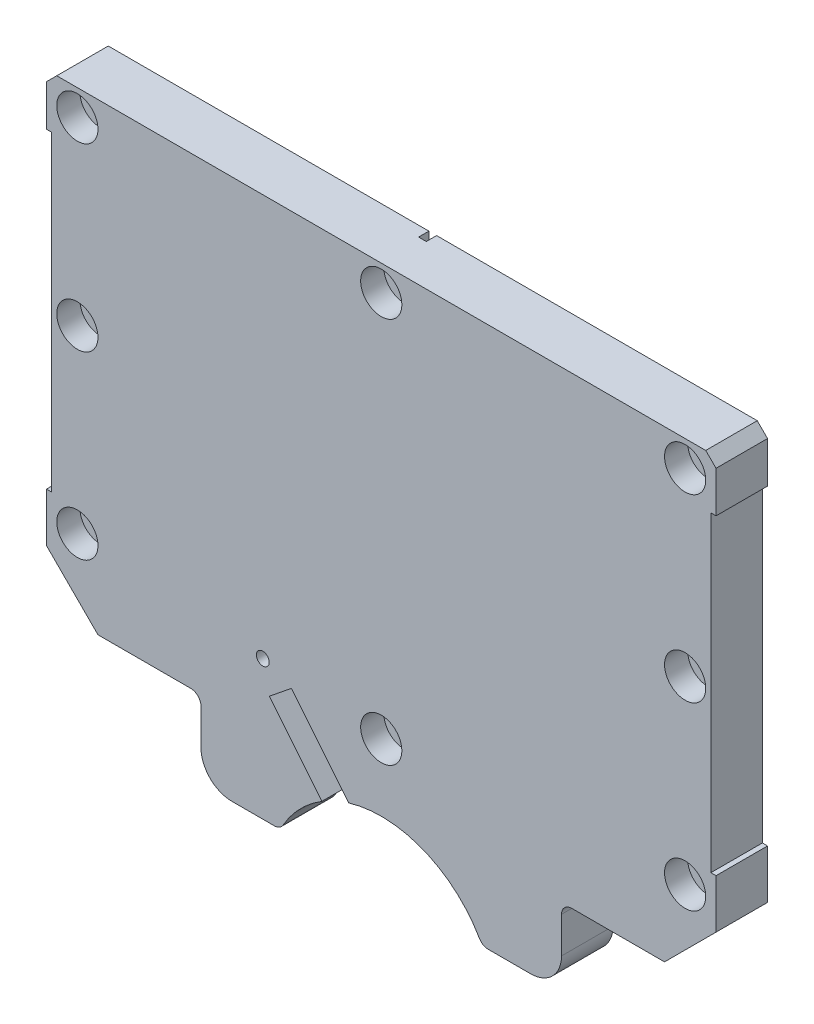
from build123d import *

# Parameters (mm, degrees)
SKETCH1_W                                            = 130
SKETCH1_H                                            = 105
BOSS_EXTRUDE1_DEPTH                                  = 5
SKETCH3_R                                            = 22
CUT_EXTRUDE2_DEPTH                                   = 85.150163399
SKETCH7_W                                            = 30
SKETCH7_H                                            = 10
CUT_EXTRUDE5_DEPTH                                   = 15
FILLET1_R                                            = 6
CHAMFER1_SIZE                                        = 10
FILLET2_R                                            = 2
CUT_EXTRUDE8_DEPTH                                   = 85.150163399
FILLET3_R                                            = 2
CHAMFER2_SIZE                                        = 2
SKETCH15_W                                           = 1
SKETCH15_H                                           = 60.5
CUT_EXTRUDE10_DEPTH                                  = 85.150163399
HOLE_SIZE_PER_SOCKET_HEAD_CAP_SCREW_TYPE_D           = 4.5
HOLE_SIZE_PER_SOCKET_HEAD_CAP_SCREW_TYPE_CBORE_D     = 8
HOLE_SIZE_PER_SOCKET_HEAD_CAP_SCREW_TYPE_CBORE_DEPTH = 4.5
M3_TAPPED_HOLE1_D                                    = 2.5
M3_TAPPED_HOLE1_DEPTH                                = 8.5
M3_TAPPED_HOLE1_TIP                                  = 0.751075774
SKETCH20_W                                           = 1.5
SKETCH20_H                                           = 105
CUT_EXTRUDE11_DEPTH                                  = 2


with BuildPart() as part:
    # Sketch1 → Boss-Extrude1 (new, symmetric)
    with BuildSketch(Plane.XY):
        Rectangle(SKETCH1_W, SKETCH1_H)
    extrude(amount=BOSS_EXTRUDE1_DEPTH, both=True)

    # Sketch3 → Cut-Extrude2 (cut, through all)
    with BuildSketch(Plane.XY.offset(5)):
        with Locations((0, -62.5)):
            Circle(SKETCH3_R)
    extrude(amount=-CUT_EXTRUDE2_DEPTH, mode=Mode.SUBTRACT)

    # Sketch7 → Cut-Extrude5 (cut)
    with BuildSketch(Plane.XZ.offset(52.5)):
        with Locations((-50, 0)):
            Rectangle(SKETCH7_W, SKETCH7_H)
        with Locations((50, 0)):
            Rectangle(SKETCH7_W, SKETCH7_H)
    extrude(amount=-CUT_EXTRUDE5_DEPTH, mode=Mode.SUBTRACT)

    # Fillet1
    fillet1_edges = [part.edges().sort_by_distance(p)[0] for p in [
        (-35, -52.5, 0),
        (35, -52.5, 0),
    ]]
    fillet(fillet1_edges, radius=FILLET1_R)

    # Chamfer1
    chamfer1_edges = [part.edges().sort_by_distance(p)[0] for p in [
        (-65, -37.5, 0),
        (65, -37.5, 0),
    ]]
    chamfer(chamfer1_edges, length=CHAMFER1_SIZE)

    # Fillet2
    fillet2_edges = [part.edges().sort_by_distance(p)[0] for p in [
        (-35, -37.5, 0),
        (35, -37.5, 0),
    ]]
    fillet(fillet2_edges, radius=FILLET2_R)

    # Sketch10 → Cut-Extrude8 (cut, through all)
    with BuildSketch(Plane.XY.offset(5)):
        Polygon((-21.710710609, -31.184123297), (-17.436407821, -27.722861146), (-4.85, -43.265780375), (-9.124302788, -46.727042526), align=None)
    extrude(amount=-CUT_EXTRUDE8_DEPTH, mode=Mode.SUBTRACT)

    # Fillet3
    fillet3_edges = [part.edges().sort_by_distance(p)[0] for p in [
        (-19.595917942, -52.5, 0),
        (19.595917942, -52.5, 0),
    ]]
    fillet(fillet3_edges, radius=FILLET3_R)

    # Chamfer2
    chamfer2_edges = [part.edges().sort_by_distance(p)[0] for p in [
        (-65, 52.5, 0),
        (65, 52.5, 0),
    ]]
    chamfer(chamfer2_edges, length=CHAMFER2_SIZE)

    # Sketch15 → Cut-Extrude10 (cut, through all)
    with BuildSketch(Plane(origin=(0, 0, -5), x_dir=(-1, 0, 0), z_dir=(0, 0, -1))):
        with Locations((-64.5, 12.25)):
            Rectangle(SKETCH15_W, SKETCH15_H)
        with Locations((64.5, 12.25)):
            Rectangle(SKETCH15_W, SKETCH15_H)
    extrude(amount=-CUT_EXTRUDE10_DEPTH, mode=Mode.SUBTRACT)

    # Hole size per socket head cap screw type 0 (through all)
    with Locations(Plane.XY.offset(5)):
        with Locations((59, 47.5), (0, 47.5), (-59, 47.5), (-59, 12.5), (-59, -22.5), (0, -27.5), (59, -22.5), (59, 12.5)):
            CounterBoreHole(HOLE_SIZE_PER_SOCKET_HEAD_CAP_SCREW_TYPE_D / 2, HOLE_SIZE_PER_SOCKET_HEAD_CAP_SCREW_TYPE_CBORE_D / 2, HOLE_SIZE_PER_SOCKET_HEAD_CAP_SCREW_TYPE_CBORE_DEPTH)

    # M3 Tapped Hole1
    with Locations(Plane.XY.offset(5)):
        with Locations((-23, -25.5)):
            Hole(M3_TAPPED_HOLE1_D / 2, depth=M3_TAPPED_HOLE1_DEPTH)
            with Locations((0, 0, -(M3_TAPPED_HOLE1_DEPTH + M3_TAPPED_HOLE1_TIP / 2))):  # 118° drill point
                Cone(0, M3_TAPPED_HOLE1_D / 2, M3_TAPPED_HOLE1_TIP, mode=Mode.SUBTRACT)

    # Sketch20 → Cut-Extrude11 (cut)
    with BuildSketch(Plane(origin=(0, 0, -5), x_dir=(-1, 0, 0), z_dir=(0, 0, -1))):
        Rectangle(SKETCH20_W, SKETCH20_H)
    extrude(amount=-CUT_EXTRUDE11_DEPTH, mode=Mode.SUBTRACT)


solid = part.part
